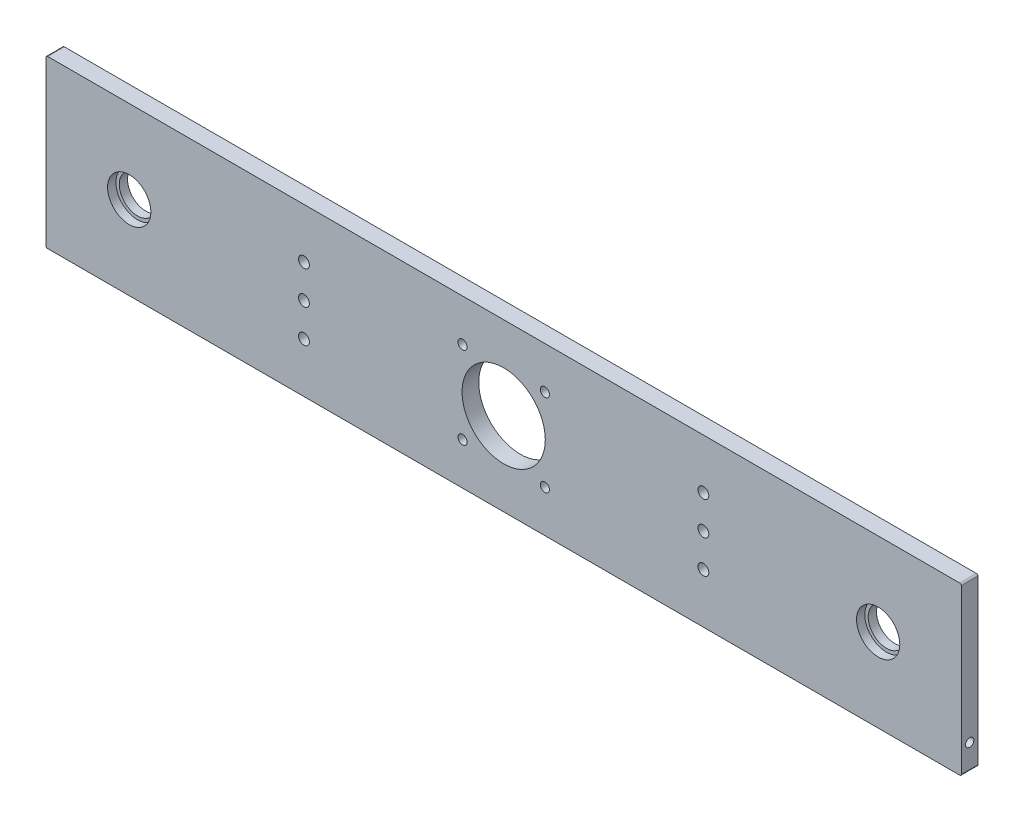
from build123d import *

# Parameters (mm, degrees)
SKETCH1_W           = 550
SKETCH1_H           = 100
BOSS_EXTRUDE1_DEPTH = 10
SKETCH3_R           = 13
CUT_EXTRUDE2_DEPTH  = 5
SKETCH4_R           = 11
CUT_EXTRUDE3_DEPTH  = 280.55321497
SKETCH5_R           = 25
CUT_EXTRUDE4_DEPTH  = 280.687325419
SKETCH6_R           = 2.75
CUT_EXTRUDE5_DEPTH  = 280.687325419
SKETCH7_R           = 3.25
CUT_EXTRUDE6_DEPTH  = 280.687325419
FILLET1_R           = 1


with BuildPart() as part:
    # Sketch1 → Boss-Extrude1 (new body)
    with BuildSketch(Plane.XY):
        Rectangle(SKETCH1_W, SKETCH1_H)
    extrude(amount=BOSS_EXTRUDE1_DEPTH)

    # Sketch3 → Cut-Extrude2 (cut)
    with BuildSketch(Plane.XY.offset(10)):
        with Locations((225, 0)):
            Circle(SKETCH3_R)
        with Locations(Location((-225, 0, 0), (0, 0, 180))):
            Circle(SKETCH3_R)
    extrude(amount=-CUT_EXTRUDE2_DEPTH, mode=Mode.SUBTRACT)

    # Sketch4 → Cut-Extrude3 (cut, through all)
    with BuildSketch(Plane.XY.offset(5)):
        with Locations((225, 0)):
            Circle(SKETCH4_R)
        with Locations(Location((-225, 0, 0), (0, 0, 180))):
            Circle(SKETCH4_R)
    extrude(amount=-CUT_EXTRUDE3_DEPTH, mode=Mode.SUBTRACT)

    # Sketch5 → Cut-Extrude4 (cut, through all)
    with BuildSketch(Plane.XY.offset(10)):
        Circle(SKETCH5_R)
    extrude(amount=-CUT_EXTRUDE4_DEPTH, mode=Mode.SUBTRACT)

    # Sketch6 → Cut-Extrude5 (cut, through all)
    with BuildSketch(Plane.XY.offset(10)):
        with Locations((-24.748737342, 24.748737342)):
            Circle(SKETCH6_R)
        with Locations((24.748737342, 24.748737342)):
            Circle(SKETCH6_R)
        with Locations((24.748737342, -24.748737342)):
            Circle(SKETCH6_R)
        with Locations((-24.748737342, -24.748737342)):
            Circle(SKETCH6_R)
    extrude(amount=-CUT_EXTRUDE5_DEPTH, mode=Mode.SUBTRACT)

    # Sketch7 → Cut-Extrude6 (cut, through all)
    with BuildSketch(Plane.XY.offset(10)):
        with Locations((-120, -20)):
            Circle(SKETCH7_R)
        with Locations((120, -20)):
            Circle(SKETCH7_R)
        with Locations((120, 20)):
            Circle(SKETCH7_R)
        with Locations((-120, 20)):
            Circle(SKETCH7_R)
        with Locations((-120, 0)):
            Circle(SKETCH7_R)
        with Locations((120, 0)):
            Circle(SKETCH7_R)
    extrude(amount=-CUT_EXTRUDE6_DEPTH, mode=Mode.SUBTRACT)

    # Fillet1
    fillet1_edges = [part.edges().sort_by_distance(p)[0] for p in [
        (-275, 50, 5),
        (275, 50, 5),
        (275, -50, 5),
        (-275, -50, 5),
    ]]
    fillet(fillet1_edges, radius=FILLET1_R)

    # Sketch9 → M6 Tapped Hole1 (revolve, cut)
    with BuildSketch(Plane(origin=(-275, -35, 5), x_dir=(0, 0, 1), z_dir=(0, 1, 0))):
        Polygon((0, 0), (0, 19.502151548), (2.5, 18), (2.5, 0), align=None)
    m6_tapped_hole1 = revolve(axis=Axis((-281.35, -35, 5), (1, 0, 0)), mode=Mode.SUBTRACT)

    # Mirror1: M6 Tapped Hole1 across plane
    add(m6_tapped_hole1.mirror(Plane(origin=(0, 0, 0), x_dir=(0, 0, 1), z_dir=(1, 0, 0))), mode=Mode.SUBTRACT)


solid = part.part
